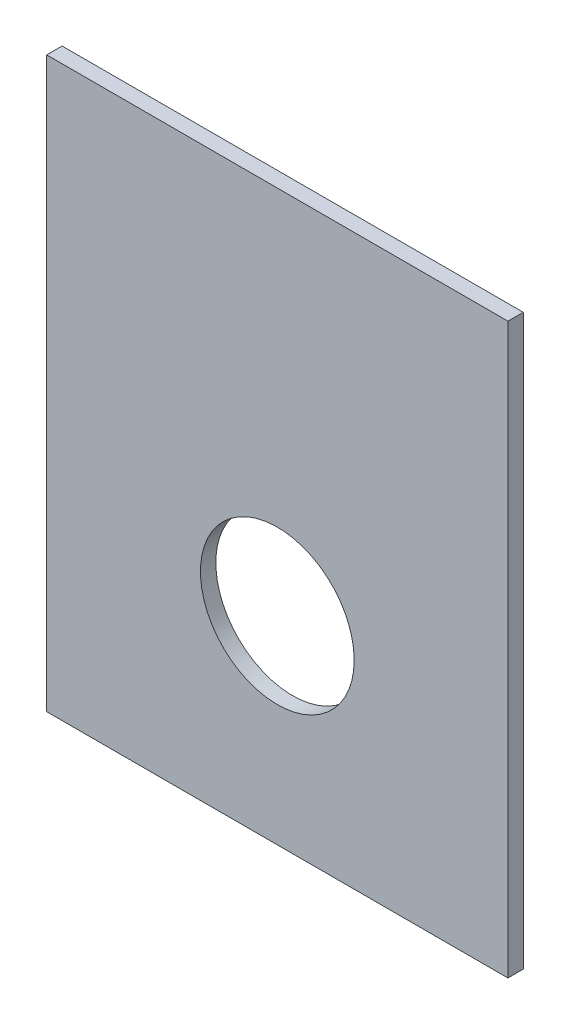
from build123d import *

# Parameters (mm, degrees)
SKETCH1_W           = 300
SKETCH1_H           = 370
SKETCH1_R           = 50
BOSS_EXTRUDE1_DEPTH = 10


with BuildPart() as part:
    # Sketch1 → Boss-Extrude1 (new body)
    with BuildSketch(Plane.XY):
        with Locations((150, 185)):
            Rectangle(SKETCH1_W, SKETCH1_H)
        with Locations((150, 129)):
            Circle(SKETCH1_R, mode=Mode.SUBTRACT)
    extrude(amount=BOSS_EXTRUDE1_DEPTH)


solid = part.part
